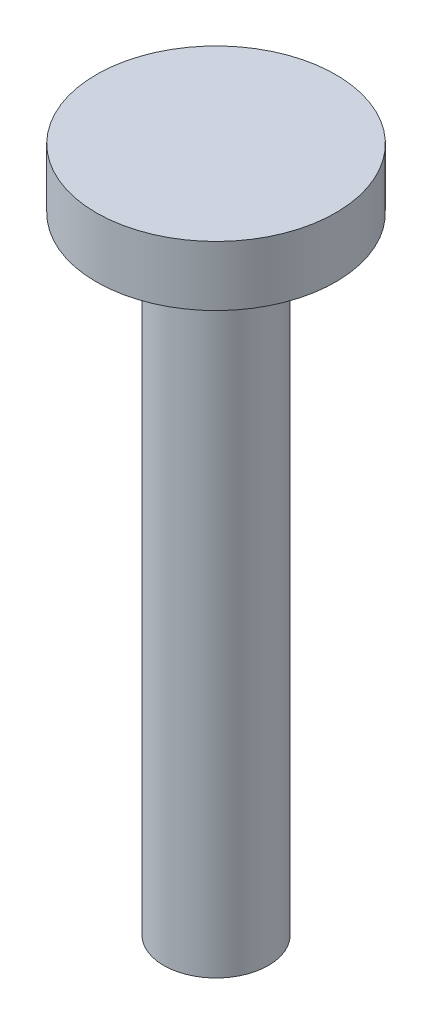
SolidWorks part; units mm, degrees
ref_plane "Front Plane" through (0, 0, 0) normal (0, 0, 1) x (1, 0, 0)
ref_plane "Top Plane" through (0, 0, 0) normal (0, 1, 0) x (1, 0, 0)
ref_plane "Right Plane" through (0, 0, 0) normal (1, 0, 0) x (0, 0, -1)
other "Configuration Table"
sketch "Sketch1" plane through (0, 0, 0) normal (0, 0, 1) x (1, 0, 0)
  line L0 (0, -30) -> (0, 30) construction
  line L1 (0, 30) -> (4, 30)
  line L2 (4, 30) -> (4, 28)
  line L3 (4, 28) -> (1.75, 27.1005)
  line L4 (1.75, 27.1005) -> (1.75, 7.1005)
  line L5 (1.75, 7.1005) -> (0, 7.1005)
  line L6 (0, 30) -> (0, 7.1005)
  point P4 (0, 0)
  dimension "D1" = 4
  dimension "D2" = 2
  dimension "D3" = 20
  dimension "D4" = 1.75
revolve "Revolve1" add sketch "Sketch1" angle 360 about L6
